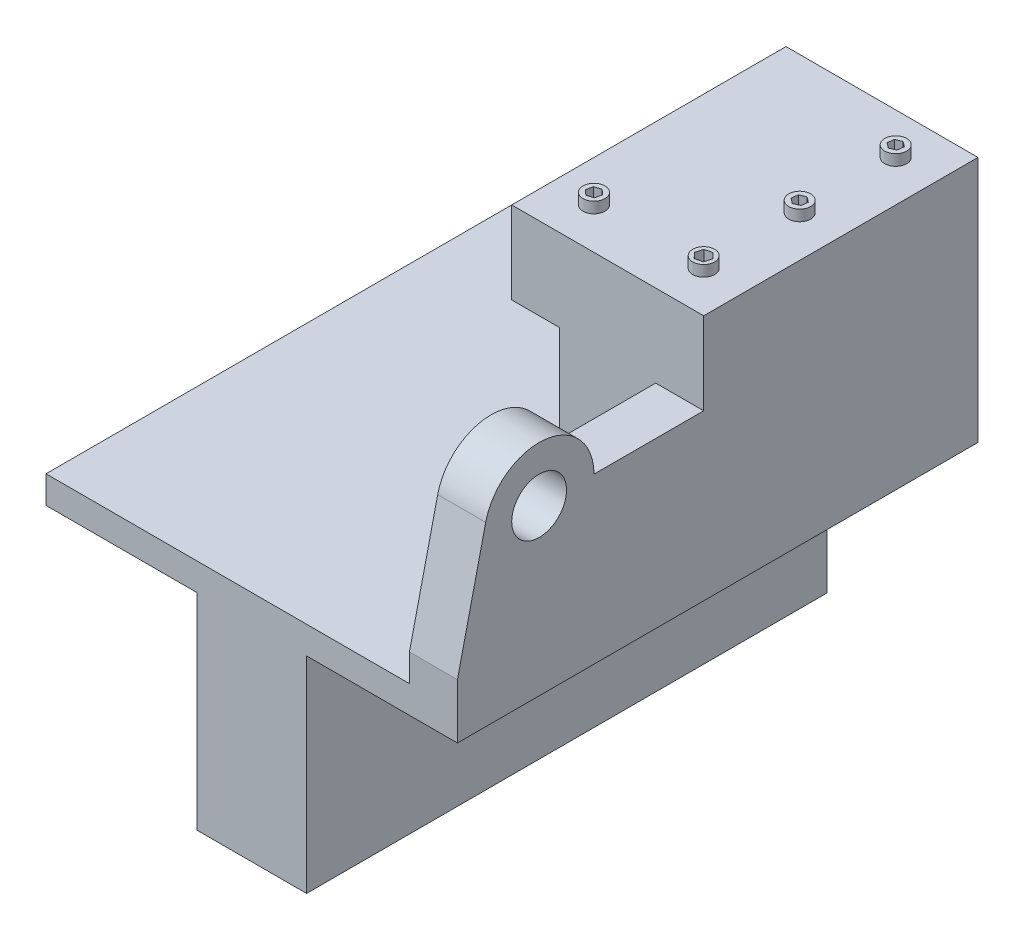
from build123d import *

# Parameters (mm, degrees)
SKETCH1_W           = 70
SKETCH1_H           = 100
BOSS_EXTRUDE1_DEPTH = 30
SKETCH2_R           = 4
BOSS_EXTRUDE2_DEPTH = 4
SKETCH3_W           = 35
SKETCH3_H           = 100
BOSS_EXTRUDE3_DEPTH = 40
SKETCH4_R           = 10
BOSS_EXTRUDE4_DEPTH = 17.5
BOSS_EXTRUDE5_DEPTH = 10
SKETCH6_W           = 150
SKETCH6_H           = 189.781220368
BOSS_EXTRUDE6_DEPTH = 10
SKETCH7_W           = 40
SKETCH7_H           = 189.781220368
BOSS_EXTRUDE7_DEPTH = 75


with BuildPart() as part:
    # Sketch1 → Boss-Extrude1 (new body)
    with BuildSketch(Plane(origin=(0, 0, 0), x_dir=(1, 0, 0), z_dir=(0, 1, 0))):
        Rectangle(SKETCH1_W, SKETCH1_H)
    extrude(amount=BOSS_EXTRUDE1_DEPTH)

    # Sketch2 → Boss-Extrude2 (add)
    # profile 1 of 4: a face of its own
    with BuildSketch(Plane(origin=(0, 30, 0), x_dir=(1, 0, 0), z_dir=(0, 1, 0))):
        with Locations(Location((-20, -35, 0), (0, 0, 270))):
            Circle(SKETCH2_R)
        Polygon((-18.132531053, -36.656757487), (-17.631471454, -34.211103194), (-19.498940402, -32.554345707), (-21.867468947, -33.343242513), (-22.368528546, -35.788896806), (-20.501059598, -37.445654293), align=None, mode=Mode.SUBTRACT)
    # profile 2 of 4: a face of its own
    with BuildSketch(Plane(origin=(0, 30, 0), x_dir=(1, 0, 0), z_dir=(0, 1, 0))):
        with Locations(Location((20, -35, 0), (0, 0, 270))):
            Circle(SKETCH2_R)
        Polygon((21.913058762, -37.035169602), (22.719037957, -34.360827314), (20.805979195, -32.325657712), (18.086941238, -32.964830398), (17.280962043, -35.639172686), (19.194020805, -37.674342288), align=None, mode=Mode.SUBTRACT)
    # profile 3 of 4: a face of its own
    with BuildSketch(Plane(origin=(0, 30, 0), x_dir=(1, 0, 0), z_dir=(0, 1, 0))):
        with Locations(Location((20, 0, 0), (0, 0, 270))):
            Circle(SKETCH2_R)
        Polygon((21.913058762, -1.47020522), (22.229764451, 0.921654877), (20.316705689, 2.391860097), (18.086941238, 1.47020522), (17.770235549, -0.921654877), (19.683294311, -2.391860097), align=None, mode=Mode.SUBTRACT)
    # profile 4 of 4: a face of its own
    with BuildSketch(Plane(origin=(0, 30, 0), x_dir=(1, 0, 0), z_dir=(0, 1, 0))):
        with Locations(Location((20, 35, 0), (0, 0, 270))):
            Circle(SKETCH2_R)
        Polygon((21.913058762, 33.534680981), (22.225532876, 35.924097978), (20.312474114, 37.389416996), (18.086941238, 36.465319019), (17.774467124, 34.075902022), (19.687525886, 32.610583004), align=None, mode=Mode.SUBTRACT)
    extrude(amount=BOSS_EXTRUDE2_DEPTH)

    # Sketch3 → Boss-Extrude3 (add)
    with BuildSketch(Plane.XZ):
        Rectangle(SKETCH3_W, SKETCH3_H)
    extrude(amount=BOSS_EXTRUDE3_DEPTH)

    # Sketch4 → Boss-Extrude4 (add)
    with BuildSketch(Plane(origin=(17.5, 0, 0), x_dir=(0, 0, -1), z_dir=(1, 0, 0))):
        with BuildLine():
            Line((-50, -40), (-139.781220368, -40))
            Line((-139.781220368, -40), (-129.48544067, 4.507505064))
            ThreePointArc((-129.48544067, 4.507505064), (-107.731609976, 19.87094378), (-90, 0))
            Line((-90, 0), (-50, 0))
            Line((-50, 0), (50, 0))
            Line((50, 0), (50, -40))
            Line((50, -40), (-50, -40))
        make_face()
        with Locations(Location((-110, 0, 0), (0, 0, 180))):
            Circle(SKETCH4_R, mode=Mode.SUBTRACT)
    extrude(amount=BOSS_EXTRUDE4_DEPTH)

    # Sketch5 → Boss-Extrude5 (add)
    with BuildSketch(Plane.XZ.offset(40)):
        Polygon((17.5, 139.781220368), (35, 139.781220368), (35, -50), (-17.5, -50), (-17.5, 50), (17.5, 50), align=None)
    extrude(amount=BOSS_EXTRUDE5_DEPTH)

    # Sketch6 → Boss-Extrude6 (add)
    with BuildSketch(Plane.XZ.offset(50)):
        with Locations((-40, 44.890610184)):
            Rectangle(SKETCH6_W, SKETCH6_H)
    extrude(amount=BOSS_EXTRUDE6_DEPTH)

    # Sketch7 → Boss-Extrude7 (add)
    with BuildSketch(Plane.XZ.offset(60)):
        with Locations((-40, 44.890610184)):
            Rectangle(SKETCH7_W, SKETCH7_H)
    extrude(amount=BOSS_EXTRUDE7_DEPTH)


solid = part.part
